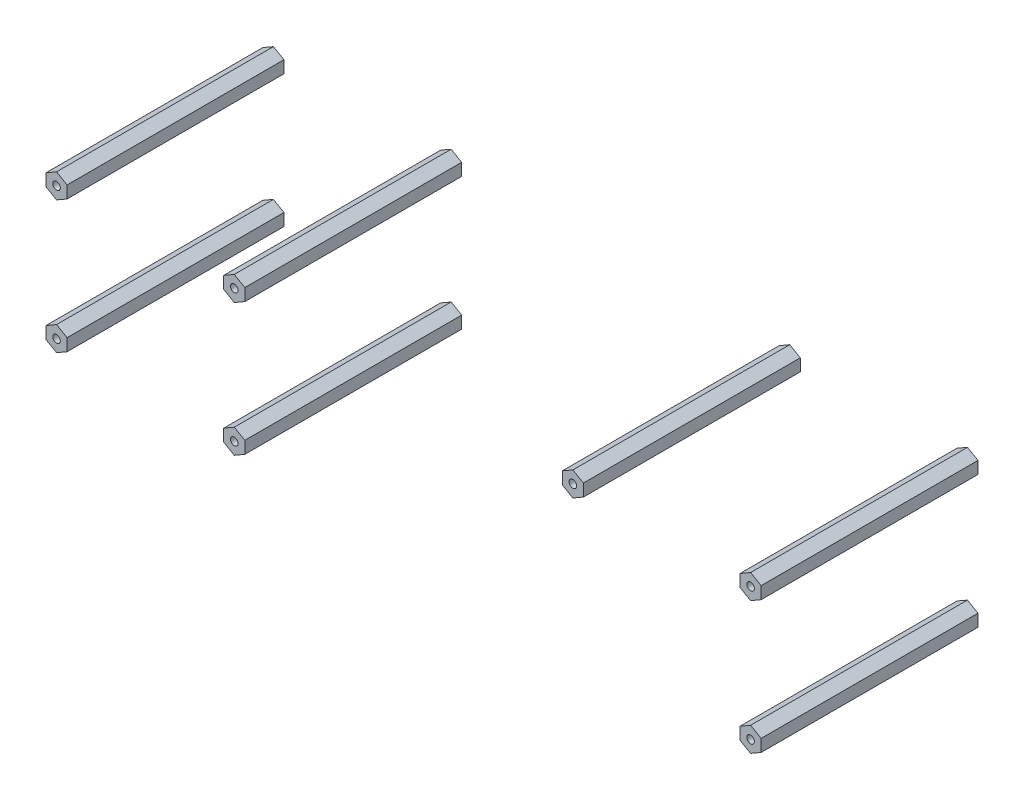
SolidWorks part; units mm, degrees
ref_plane "Front Plane" through (0, 0, 0) normal (0, 0, 1) x (1, 0, 0)
ref_plane "Top Plane" through (0, 0, 0) normal (0, 1, 0) x (1, 0, 0)
ref_plane "Right Plane" through (0, 0, 0) normal (1, 0, 0) x (0, 0, -1)
other "Configuration Table"
sketch "Sketch1" plane through (0, 0, 0) normal (0, 0, 1) x (1, 0, 0)
  line L0 (125, -87) -> (125, 27) construction
  line L1 (118.7, -6.0207) -> (115.2, -4)
  line L2 (115.2, -4) -> (111.7, -6.0207)
  line L3 (111.7, -6.0207) -> (111.7, -10.0622)
  line L4 (111.7, -10.0622) -> (115.2, -12.0829)
  line L5 (115.2, -12.0829) -> (118.7, -10.0622)
  line L6 (118.7, -10.0622) -> (118.7, -6.0207)
  line L7 (78, 30) -> (122, 30) construction
  line L8 (125, -30) -> (-18.7468, -30) construction
  line L10 (59.7, -6.0207) -> (56.2, -4)
  line L11 (56.2, -4) -> (52.7, -6.0207)
  line L12 (52.7, -6.0207) -> (52.7, -10.0622)
  line L13 (52.7, -10.0622) -> (56.2, -12.0829)
  line L14 (56.2, -12.0829) -> (59.7, -10.0622)
  line L15 (59.7, -10.0622) -> (59.7, -6.0207)
  line L21 (118.7, -49.9378) -> (118.7, -53.9793)
  line L22 (115.2, -47.9171) -> (118.7, -49.9378)
  line L23 (111.7, -49.9378) -> (115.2, -47.9171)
  line L24 (111.7, -53.9793) -> (111.7, -49.9378)
  line L25 (115.2, -56) -> (111.7, -53.9793)
  line L26 (118.7, -53.9793) -> (115.2, -56)
  line L27 (0, 0) -> (0, -61.6069) construction
  line L28 (-118.7, -53.9793) -> (-115.2, -56)
  line L29 (-115.2, -56) -> (-111.7, -53.9793)
  line L30 (-111.7, -53.9793) -> (-111.7, -49.9378)
  line L31 (-111.7, -49.9378) -> (-115.2, -47.9171)
  line L32 (-115.2, -47.9171) -> (-118.7, -49.9378)
  line L33 (-118.7, -49.9378) -> (-118.7, -53.9793)
  line L34 (-118.7, -10.0622) -> (-118.7, -6.0207)
  line L35 (-115.2, -12.0829) -> (-118.7, -10.0622)
  line L36 (-111.7, -10.0622) -> (-115.2, -12.0829)
  line L37 (-111.7, -6.0207) -> (-111.7, -10.0622)
  line L38 (-115.2, -4) -> (-111.7, -6.0207)
  line L39 (-118.7, -6.0207) -> (-115.2, -4)
  line L46 (-59.7, -10.0622) -> (-59.7, -6.0207)
  line L47 (-56.2, -12.0829) -> (-59.7, -10.0622)
  line L48 (-52.7, -10.0622) -> (-56.2, -12.0829)
  line L49 (-52.7, -6.0207) -> (-52.7, -10.0622)
  line L50 (-56.2, -4) -> (-52.7, -6.0207)
  line L51 (-59.7, -6.0207) -> (-56.2, -4)
  line L52 (-59.7, -53.9793) -> (-56.2, -56)
  line L53 (-56.2, -56) -> (-52.7, -53.9793)
  line L54 (-52.7, -53.9793) -> (-52.7, -49.9378)
  line L55 (-52.7, -49.9378) -> (-56.2, -47.9171)
  line L56 (-56.2, -47.9171) -> (-59.7, -49.9378)
  line L57 (-59.7, -49.9378) -> (-59.7, -53.9793)
  circle A0 centre (115.2, -8.0415) radius 3.5 construction
  circle A1 centre (56.2, -8.0415) radius 3.5 construction
  circle A3 centre (115.2, -51.9585) radius 3.5 construction
  circle A4 centre (-115.2, -51.9585) radius 3.5 construction
  circle A5 centre (-115.2, -8.0415) radius 3.5 construction
  circle A6 centre (-115.2, -51.9585) radius 3.5 construction
  circle A8 centre (-56.2, -8.0415) radius 3.5 construction
  circle A9 centre (-56.2, -51.9585) radius 3.5 construction
  dimension "D1" = 6.3
  dimension "D2" = 34
  dimension "D3" = 7
  dimension "D4" = 52
  dimension "D5" = 7
extrude "Boss-Extrude1" add sketch "Sketch1" along normal blind 70 and the other way blind 2
hole_wizard "M3 Tapped Hole1" positions "Sketch2" profile "Sketch3" tap size "M3" standard "GB"
sketch "Sketch2" plane through (0, 0, 70) normal (0, 0, 1) x (1, 0, 0)
  point P0 (-115.2, -52)
  point P3 (-115.2, -8)
  point P6 (-56.2, -8)
  point P9 (-56.2, -52)
  point P12 (56.2, -8)
  point P15 (115.2, -8)
  point P18 (115.2, -52)
sketch "Sketch3" plane through (-115.2, -52, 70) normal (1, 0, 0) x (0, -1, 0)
  line L0 (0, 0) -> (0, 9.2511)
  line L1 (0, 9.2511) -> (1.25, 8.5)
  line L2 (1.25, 8.5) -> (1.25, 0)
  line L5 (1.25, 0) -> (0, 0)
  line L10 (0, 9.2511) -> (-1.25, 8.5) construction
  line L11 (0, -6.35) -> (0, 107.95) construction
  dimension "螺纹孔钻头直径" = 2.5
  dimension "螺纹孔钻头深度" = 8.5
  dimension "导头角度" = 118
cosmetic thread "Cosmetic Thread1" parameters "D1"=6, "D2"=3
cosmetic thread "Cosmetic Thread2" parameters "D1"=6, "D2"=3
cosmetic thread "Cosmetic Thread3" parameters "D1"=6, "D2"=3
cosmetic thread "Cosmetic Thread4" parameters "D1"=6, "D2"=3
cosmetic thread "Cosmetic Thread5" parameters "D1"=6, "D2"=3
cosmetic thread "Cosmetic Thread6" parameters "D1"=6, "D2"=3
cosmetic thread "Cosmetic Thread7" parameters "D1"=6, "D2"=3
